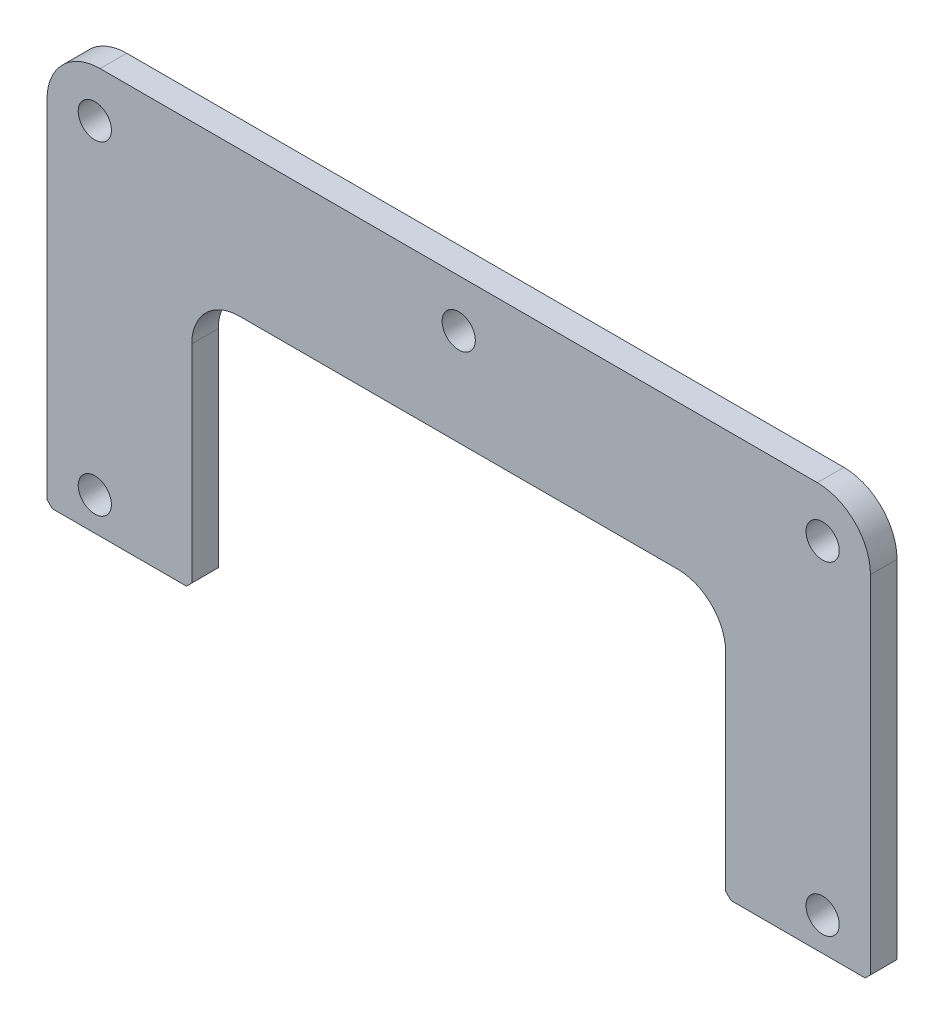
SolidWorks part; units mm, degrees
material "20Mn"
ref_plane "前视基准面" through (0, 0, 0) normal (0, 0, 1) x (1, 0, 0)
ref_plane "上视基准面" through (0, 0, 0) normal (0, 1, 0) x (1, 0, 0)
ref_plane "右视基准面" through (0, 0, 0) normal (1, 0, 0) x (0, 0, -1)
sketch "草图1" plane through (0, 0, 0) normal (0, 0, 1) x (1, 0, 0)
  line L0 (0, 0) -> (-155, 0) construction
  line L1 (-82.5, 100.5) -> (82.5, 100.5)
  line L2 (-100.5, 82.5) -> (-100.5, 2.5)
  line L3 (-82.5, -100.5) -> (82.5, -100.5) construction
  line L4 (100.5, 82.5) -> (100.5, 2.5)
  line L5 (-100.5, 100.5) -> (100.5, -100.5) construction
  line L6 (-100.5, -100.5) -> (100.5, 100.5) construction
  line L7 (-135, -155) -> (135, -155) construction
  line L8 (-155, -135) -> (-155, 0) construction
  line L9 (-135, 155) -> (135, 155)
  line L10 (155, -135) -> (155, 0) construction
  line L11 (-155, -155) -> (155, 155) construction
  line L12 (-155, 155) -> (155, -155) construction
  line L13 (0, 0) -> (155, 0) construction
  line L14 (-100.5, 2.5) -> (-155, 2.5)
  line L15 (-100.5, 2.5) -> (100.5, 2.5) construction
  line L16 (100.5, 2.5) -> (155, 2.5)
  line L17 (-155, 2.5) -> (-155, 135)
  line L18 (-100.5, 0) -> (-100.5, -82.5) construction
  line L19 (100.5, 0) -> (100.5, -82.5) construction
  line L20 (155, 2.5) -> (155, 135)
  arc A0 (-82.5, -100.5) -> (-100.5, -82.5) centre (-82.5, -82.5) cw construction
  arc A1 (82.5, -100.5) -> (100.5, -82.5) centre (82.5, -82.5) ccw construction
  arc A2 (100.5, 82.5) -> (82.5, 100.5) centre (82.5, 82.5) ccw
  arc A3 (-100.5, 82.5) -> (-82.5, 100.5) centre (-82.5, 82.5) cw
  arc A4 (135, -155) -> (155, -135) centre (135, -135) ccw construction
  arc A5 (-135, -155) -> (-155, -135) centre (-135, -135) cw construction
  arc A6 (155, 135) -> (135, 155) centre (135, 135) ccw
  arc A7 (-155, 135) -> (-135, 155) centre (-135, 135) cw
  point P0 (0, 0)
  point P18 (0, 0)
  dimension "D3" = 18
  dimension "D6" = 20
  dimension "D1" = 201
  dimension "D2" = 201
  dimension "D4" = 310
  dimension "D5" = 310
  dimension "D7" = 2.5
extrude "凸台-拉伸1" add sketch "草图1" along normal blind 10
sketch "草图2" plane through (0, 0, 10) normal (0, 0, 1) x (1, 0, 0)
  line L0 (135, 155) -> (-135, 155) construction
  line L1 (-137, -137) -> (137, -137) construction
  line L2 (-137, -137) -> (-137, 137) construction
  line L3 (-137, 137) -> (137, 137) construction
  line L4 (137, -137) -> (137, 137) construction
  line L5 (-137, -137) -> (137, 137) construction
  line L6 (-137, 137) -> (137, -137) construction
  line L8 (0, 0) -> (-137, 0) construction
  line L9 (0, 0) -> (0, 137) construction
  line L10 (155, 2.5) -> (155, 135) construction
  circle A0 centre (0, 137) radius 6.25
  circle A1 centre (0, -137) radius 6.25
  circle A2 centre (137, 0) radius 6.25 construction
  circle A3 centre (-137, 0) radius 6.25 construction
  circle A4 centre (-137, 137) radius 6.25
  circle A5 centre (137, 137) radius 6.25
  circle A6 centre (-137, -137) radius 6.25
  circle A7 centre (137, -137) radius 6.25
  circle A8 centre (-137, 15) radius 6.25
  circle A9 centre (-137, -15) radius 6.25
  circle A10 centre (137, -15) radius 6.25
  circle A11 centre (137, 15) radius 6.25
  point P0 (0, 0)
  dimension "D3" = 12.5
  dimension "D4" = 30
  dimension "D1" = 18
  dimension "D2" = 18
extrude "切除-拉伸1" cut sketch "草图2" against normal through all
chamfer "倒角1" distance 2 angle 45 4 edges at (155, 2.5, 5) (100.5, 2.5, 5) (-155, 2.5, 5) (-100.5, 2.5, 5)
